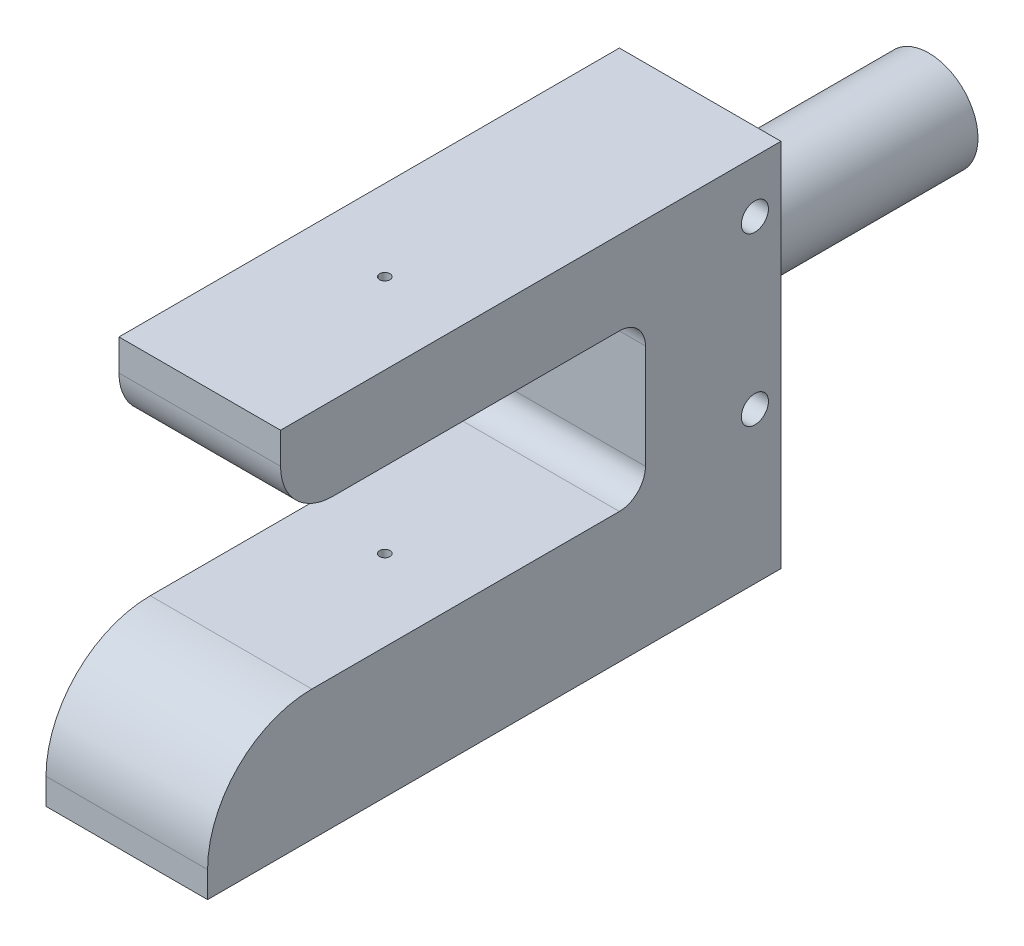
from build123d import *

# Parameters (mm, degrees)
EXTRUDE_1_DEPTH             = 31
SKETCH_2_R                  = 1
CUT_EXTRUDE_1_DEPTH         = 104.997515993
FILLET_1_R                  = 10
FILLET_2_R                  = 20
FILLET_3_R                  = 5
HOLE_WIZARD_5_2_5_2_1_D     = 5.2
HOLE_WIZARD_5_2_5_2_1_DEPTH = 63
HOLE_WIZARD_5_2_5_2_1_TIP   = 1.562237609
HOLE_WIZARD_M6_1_D          = 5
HOLE_WIZARD_M6_1_DEPTH      = 8
HOLE_WIZARD_M6_1_TIP        = 1.502151548
SKETCH_7_R                  = 9.433771821
EXTRUDE_2_DEPTH             = 44


with BuildPart() as part:
    # 草图1 → 凸台-拉伸1 (new body)
    with BuildSketch(Plane(origin=(0, 0, 0), x_dir=(0, 0, -1), z_dir=(1, 0, 0))):
        Polygon((-55.379271635, 24.957586314), (14.620728365, 24.957586314), (14.620728365, -5.042413686), (-69.379271635, -5.042413686), (-69.379271635, -30.042413686), (40.620728365, -30.042413686), (40.620728365, 40.957586314), (-55.379271635, 40.957586314), align=None)
    extrude(amount=EXTRUDE_1_DEPTH)

    # 草图2 → 切除-拉伸1 (cut, through all)
    with BuildSketch(Plane(origin=(0, 40.957586314, 0), x_dir=(1, 0, 0), z_dir=(0, 1, 0))):
        with Locations(Location((15.5, -19.879271635, 0), (0, 0, 270))):
            Circle(SKETCH_2_R)
    extrude(amount=-CUT_EXTRUDE_1_DEPTH, mode=Mode.SUBTRACT)

    # 圆角1
    fillet_1_edges = [part.edges().sort_by_distance(p)[0] for p in [
        (15.5, 24.957586314, 55.379271635),
    ]]
    fillet(fillet_1_edges, radius=FILLET_1_R)

    # 圆角2
    fillet_2_edges = [part.edges().sort_by_distance(p)[0] for p in [
        (15.5, -5.042413686, 69.379271635),
    ]]
    fillet(fillet_2_edges, radius=FILLET_2_R)

    # 圆角3
    fillet_3_edges = [part.edges().sort_by_distance(p)[0] for p in [
        (15.5, -5.042413686, -14.620728365),
        (15.5, 24.957586314, -14.620728365),
    ]]
    fillet(fillet_3_edges, radius=FILLET_3_R)

    # Ø5.2 (5.2) 直径孔1
    with Locations(Plane(origin=(31, 0, 0), x_dir=(0, 0, -1), z_dir=(1, 0, 0))):
        with Locations((35.620728365, 30.957586314), (35.620728365, -1.042413686)):
            Hole(HOLE_WIZARD_5_2_5_2_1_D / 2, depth=HOLE_WIZARD_5_2_5_2_1_DEPTH)
            with Locations((0, 0, -(HOLE_WIZARD_5_2_5_2_1_DEPTH + HOLE_WIZARD_5_2_5_2_1_TIP / 2))):  # 118° drill point
                Cone(0, HOLE_WIZARD_5_2_5_2_1_D / 2, HOLE_WIZARD_5_2_5_2_1_TIP, mode=Mode.SUBTRACT)

    # M6 螺纹孔1
    with Locations(Plane(origin=(0, 0, -40.620728365), x_dir=(-1, 0, 0), z_dir=(0, 0, -1))):
        with Locations((-15.5, -13.042413686)):
            Hole(HOLE_WIZARD_M6_1_D / 2, depth=HOLE_WIZARD_M6_1_DEPTH)
            with Locations((0, 0, -(HOLE_WIZARD_M6_1_DEPTH + HOLE_WIZARD_M6_1_TIP / 2))):  # 118° drill point
                Cone(0, HOLE_WIZARD_M6_1_D / 2, HOLE_WIZARD_M6_1_TIP, mode=Mode.SUBTRACT)

    # 草图7 → 凸台-拉伸2 (add)
    with BuildSketch(Plane(origin=(0, 0, -40.620728365), x_dir=(-1, 0, 0), z_dir=(0, 0, -1))):
        with Locations(Location((-15.370770249, 16.377500271, 0), (0, 0, 180))):
            Circle(SKETCH_7_R)
    extrude(amount=EXTRUDE_2_DEPTH)


solid = part.part
